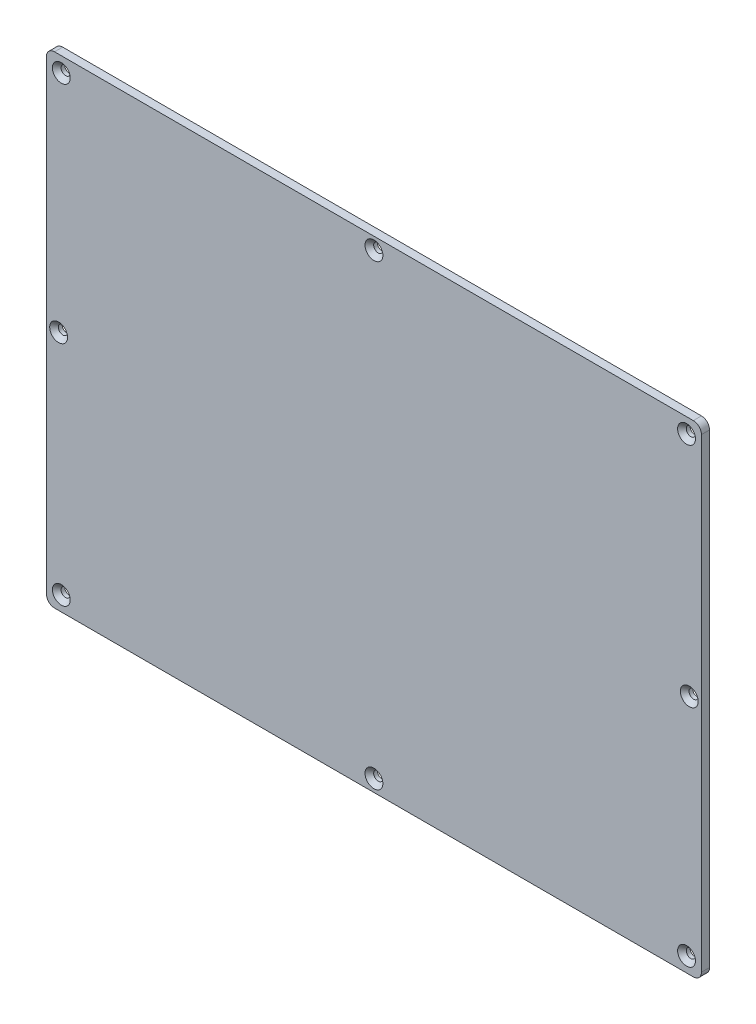
SolidWorks part; units mm, degrees
ref_plane "Front Plane" through (0, 0, 0) normal (0, 0, 1) x (1, 0, 0)
ref_plane "Top Plane" through (0, 0, 0) normal (0, 1, 0) x (1, 0, 0)
ref_plane "Right Plane" through (0, 0, 0) normal (1, 0, 0) x (0, 0, -1)
sketch "Sketch1" plane through (0, 0, 0) normal (0, 0, 1) x (1, 0, 0)
  line L1 (-121, 89) -> (121, 89)
  line L2 (-121, 89) -> (-121, -89)
  line L3 (-121, -89) -> (121, -89)
  line L4 (121, 89) -> (121, -89)
  line L5 (-121, 89) -> (121, -89) construction
  line L6 (-121, -89) -> (121, 89) construction
  point P0 (0, 0)
  dimension "D1" = 178
  dimension "D2" = 242
extrude "Boss-Extrude1" add sketch "Sketch1" along normal blind 3
fillet "Fillet1" radius 3 4 edges at (-121, -89, 1.5) (121, -89, 1.5) (121, 89, 1.5) (-121, 89, 1.5)
hole_wizard "Hole size (% per cross) for half-countersunk slotted wood screw, type 1" positions "Sketch2" profile "Sketch3" countersink size "M3" standard "GB"
sketch "Sketch2" plane through (0, 0, 3) normal (0, 0, 1) x (1, 0, 0)
  line L0 (118, 89) -> (-118, 89) construction
  line L1 (-121, 86) -> (-121, -86) construction
  line L2 (-118, -89) -> (118, -89) construction
  line L3 (121, -86) -> (121, 86) construction
  point P0 (0, 84.5)
  point P2 (-116.5, 0)
  point P4 (0, -84.5)
  point P6 (116.5, 0)
  point P17 (-115.5, 83.5)
  point P19 (-115.5, -83.5)
  point P21 (115.5, -83.5)
  point P23 (115.5, 83.5)
  dimension "D1" = 4.5
  dimension "D2" = 4.5
  dimension "D3" = 4.5
  dimension "D4" = 4.5
  dimension "D5" = 5.5
  dimension "D6" = 5.5
  dimension "D7" = 5.5
  dimension "D8" = 5.5
sketch "Sketch3" plane through (0, 84.5, 3) normal (1, 0, 0) x (0, -1, 0)
  line L0 (0, 0) -> (0, 21.0215)
  line L1 (0, 21.0215) -> (1.7, 20)
  line L2 (1.7, 20) -> (1.7, 1.6)
  line L3 (1.7, 1.6) -> (3.3, 0)
  line L5 (3.3, 0) -> (0, 0)
  line L6 (-1.7, 1.6) -> (-3.3, 0) construction
  line L10 (0, 21.0215) -> (-1.7, 20) construction
  line L11 (0, -6.35) -> (0, 107.95) construction
  dimension "孔直径" = 3.4
  dimension "孔深度" = 20
  dimension "近端锥形沉头孔直径" = 6.6
  dimension "近端锥形沉头孔角度" = 90
  dimension "导头角度" = 118
